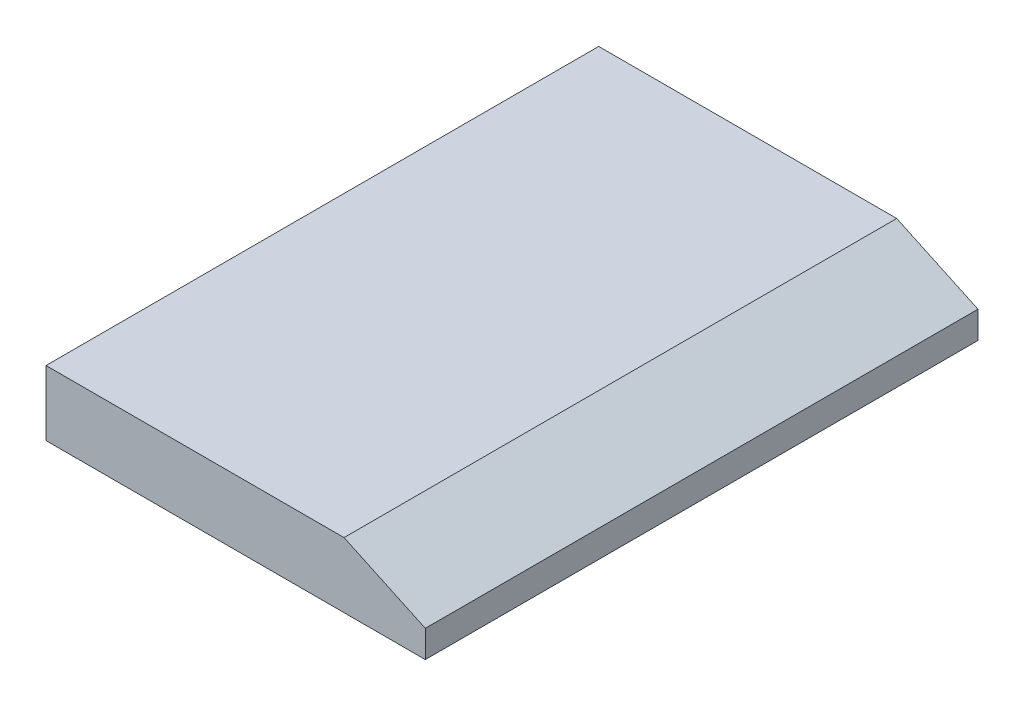
from build123d import *

# Parameters (mm, degrees)
BOSS_EXTRUDE1_DEPTH = 102


with BuildPart() as part:
    # Sketch1 → Boss-Extrude1 (new body)
    with BuildSketch(Plane.XY):
        Polygon((0, 0), (0, 5), (-15, 12), (-70, 12), (-70, 0), align=None)
    extrude(amount=BOSS_EXTRUDE1_DEPTH)


solid = part.part
